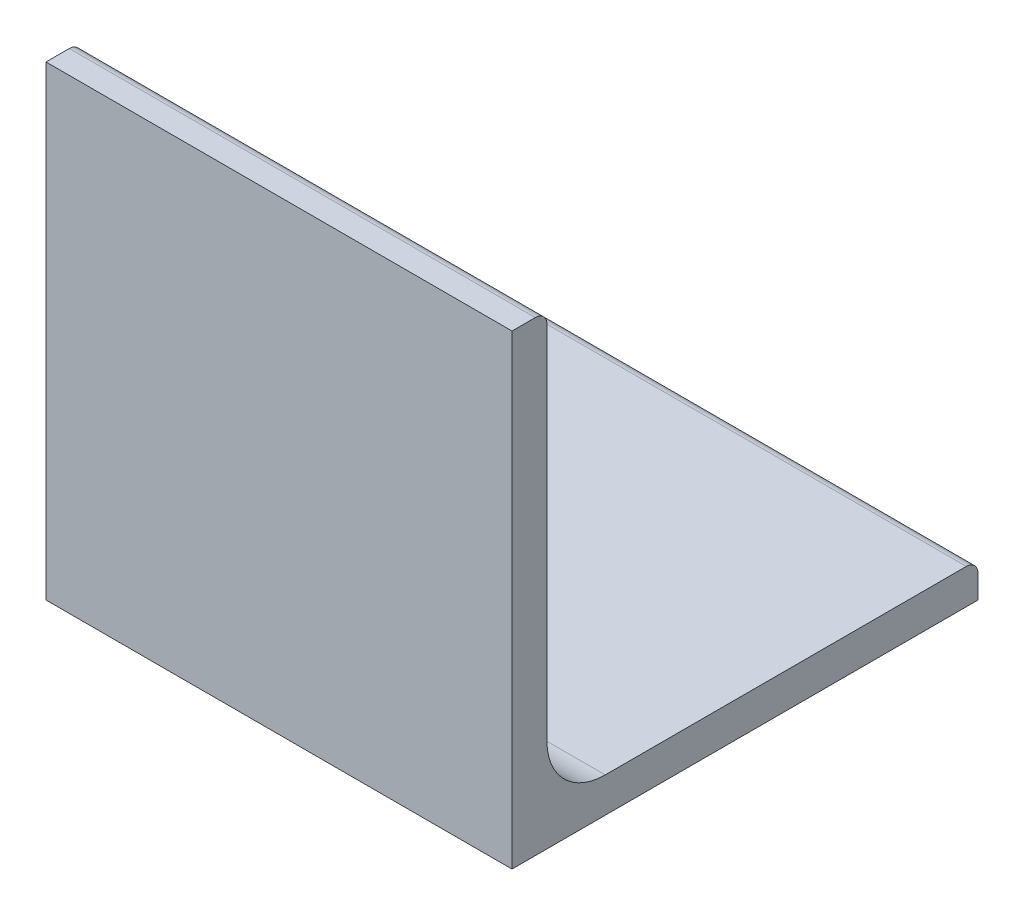
from build123d import *

# Parameters (mm, degrees)
MEMBER_40_X_3_1_DEPTH = 40


with BuildPart() as part:
    # Sketch1 → Member 40 X 3_1 (new body)
    with BuildSketch(Plane(origin=(0, 0, 0), x_dir=(0, 0, -1), z_dir=(1, 0, 0))):
        with BuildLine():
            Line((0, 0), (0, 40))
            Line((0, 40), (2, 40))
            ThreePointArc((2, 40), (2.707106781, 39.707106781), (3, 39))
            Line((3, 39), (3, 8))
            ThreePointArc((3, 8), (4.464466094, 4.464466094), (8, 3))
            Line((8, 3), (39, 3))
            ThreePointArc((39, 3), (39.707106781, 2.707106781), (40, 2))
            Line((40, 2), (40, 0))
            Line((40, 0), (0, 0))
        make_face()
    extrude(amount=MEMBER_40_X_3_1_DEPTH)


solid = part.part
